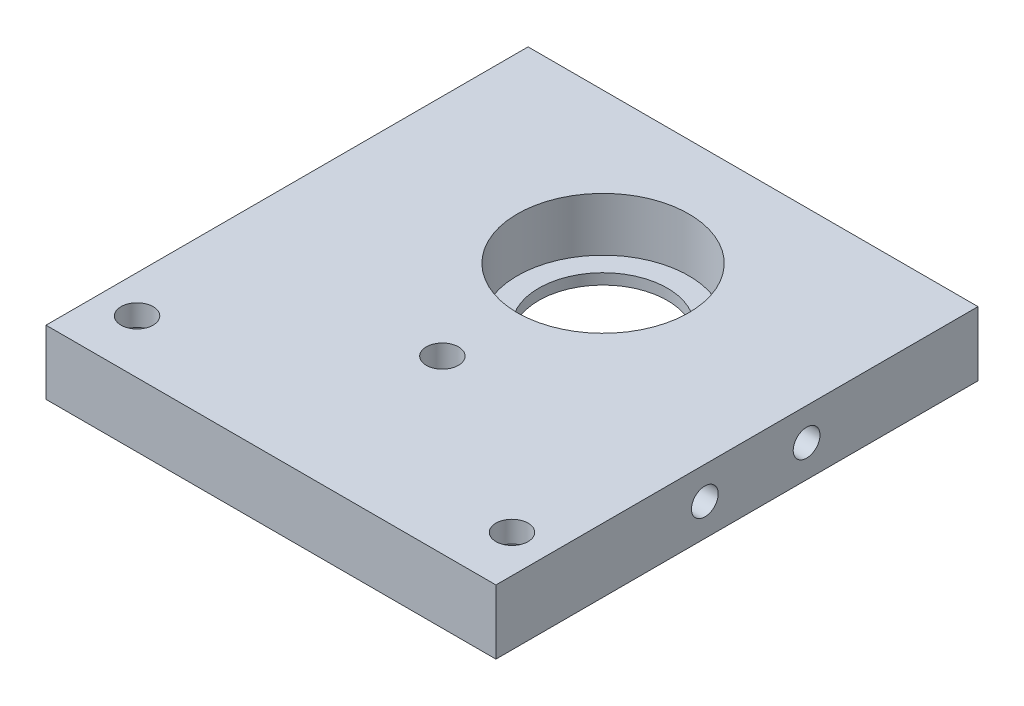
from build123d import *

# Parameters (mm, degrees)
SKETCH1_W             = 42
SKETCH1_H             = 45
SKETCH1_R             = 6
SKETCH1_R_2           = 1.5
BOSS_EXTRUDE1_DEPTH   = 6
SKETCH3_R             = 8
CUT_EXTRUDE1_DEPTH    = 5
SKETCH4_R             = 1.5
CUT_EXTRUDE2_DEPTH    = 32.356817441
SKETCH5_R             = 2.5
CUT_EXTRUDE3_DEPTH    = 4
SKETCH6_R             = 1
CUT_EXTRUDE4_DEPTH    = 2
M3_TAPPED_HOLE1_D     = 2.5
M3_TAPPED_HOLE1_DEPTH = 7.5
M3_TAPPED_HOLE1_TIP   = 0.751075774


with BuildPart() as part:
    # Sketch1 → Boss-Extrude1 (new body)
    with BuildSketch(Plane(origin=(0, 0, 0), x_dir=(1, 0, 0), z_dir=(0, 1, 0))):
        Rectangle(SKETCH1_W, SKETCH1_H)
        with Locations(Location((0, 8.5, 0), (0, 0, 270))):
            Circle(SKETCH1_R, mode=Mode.SUBTRACT)
        with Locations(Location((0, -6.5, 0), (0, 0, 270))):
            Circle(SKETCH1_R_2, mode=Mode.SUBTRACT)
    extrude(amount=BOSS_EXTRUDE1_DEPTH)

    # Sketch3 → Cut-Extrude1 (cut)
    with BuildSketch(Plane(origin=(0, 6, 0), x_dir=(1, 0, 0), z_dir=(0, 1, 0))):
        with Locations(Location((0, 8.5, 0), (0, 0, 270))):
            Circle(SKETCH3_R)
    extrude(amount=-CUT_EXTRUDE1_DEPTH, mode=Mode.SUBTRACT)

    # Sketch4 → Cut-Extrude2 (cut, through all)
    with BuildSketch(Plane(origin=(0, 6, 0), x_dir=(1, 0, 0), z_dir=(0, 1, 0))):
        with Locations(Location((-17.5, -17.5, 0), (0, 0, 270))):
            Circle(SKETCH4_R)
        with Locations(Location((17.5, -17.5, 0), (0, 0, 270))):
            Circle(SKETCH4_R)
    extrude(amount=-CUT_EXTRUDE2_DEPTH, mode=Mode.SUBTRACT)

    # Sketch5 → Cut-Extrude3 (cut)
    with BuildSketch(Plane.XZ):
        with Locations(Location((17.5, 17.5, 0), (0, 0, 270))):
            Circle(SKETCH5_R)
        with Locations(Location((-17.5, 17.5, 0), (0, 0, 270))):
            Circle(SKETCH5_R)
    extrude(amount=-CUT_EXTRUDE3_DEPTH, mode=Mode.SUBTRACT)

    # Sketch6 → Cut-Extrude4 (cut)
    with BuildSketch(Plane(origin=(21, 0, 0), x_dir=(0, 0, -1), z_dir=(1, 0, 0))):
        with Locations((6.5, 3)):
            Circle(SKETCH6_R)
        with Locations((-3, 3)):
            Circle(SKETCH6_R)
    extrude(amount=-CUT_EXTRUDE4_DEPTH, mode=Mode.SUBTRACT)

    # M3 Tapped Hole1
    with Locations(Plane(origin=(21, 0, 0), x_dir=(0, 0, -1), z_dir=(1, 0, 0))):
        with Locations((6.5, 3), (-3, 3)):
            Hole(M3_TAPPED_HOLE1_D / 2, depth=M3_TAPPED_HOLE1_DEPTH)
            with Locations((0, 0, -(M3_TAPPED_HOLE1_DEPTH + M3_TAPPED_HOLE1_TIP / 2))):  # 118° drill point
                Cone(0, M3_TAPPED_HOLE1_D / 2, M3_TAPPED_HOLE1_TIP, mode=Mode.SUBTRACT)


solid = part.part
